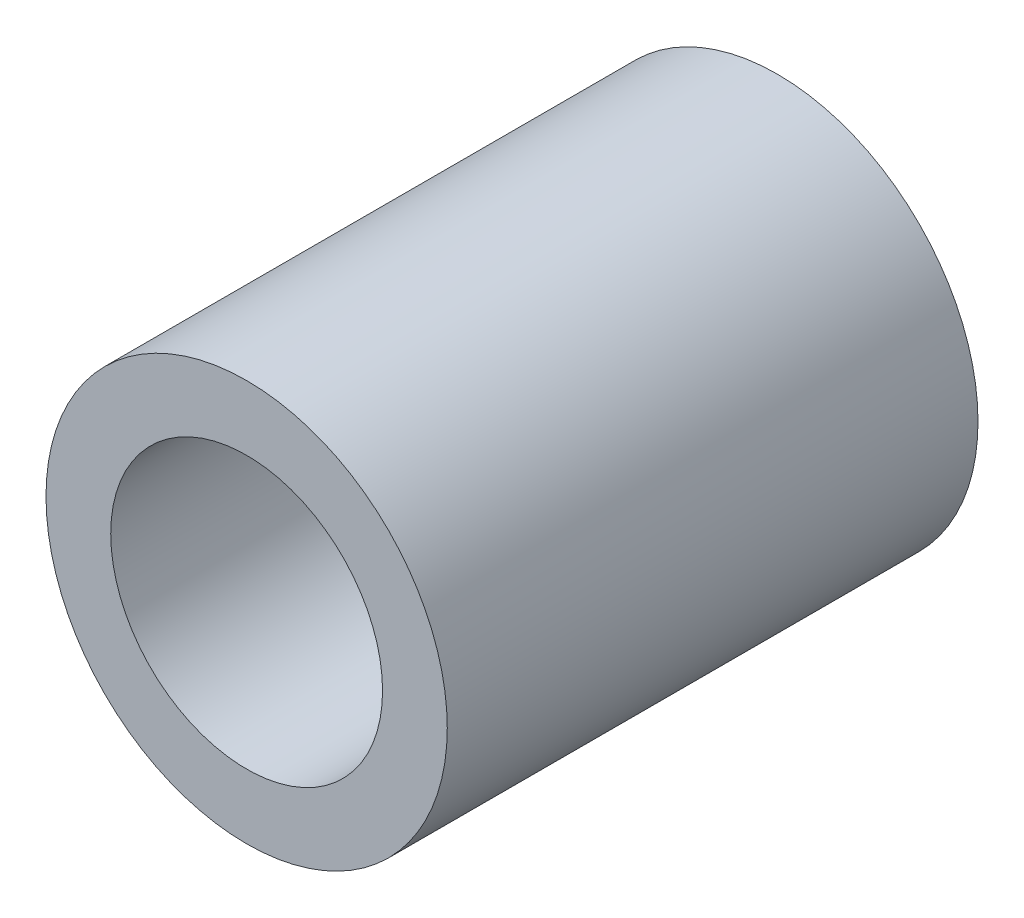
SolidWorks part; units mm, degrees
material "-"
ref_plane "Front Plane" through (0, 0, 0) normal (0, 0, 1) x (1, 0, 0)
ref_plane "Top Plane" through (0, 0, 0) normal (0, 1, 0) x (1, 0, 0)
ref_plane "Right Plane" through (0, 0, 0) normal (1, 0, 0) x (0, 0, -1)
sketch "Sketch1" plane through (0, 0, 0) normal (0, 0, 1) x (1, 0, 0)
  circle A0 centre (0, 0) radius 10.5
  circle A1 centre (0, 0) radius 15.5
  dimension "D1" = 21
  dimension "D2" = 31
extrude "Boss-Extrude1" add sketch "Sketch1" along normal blind 41
